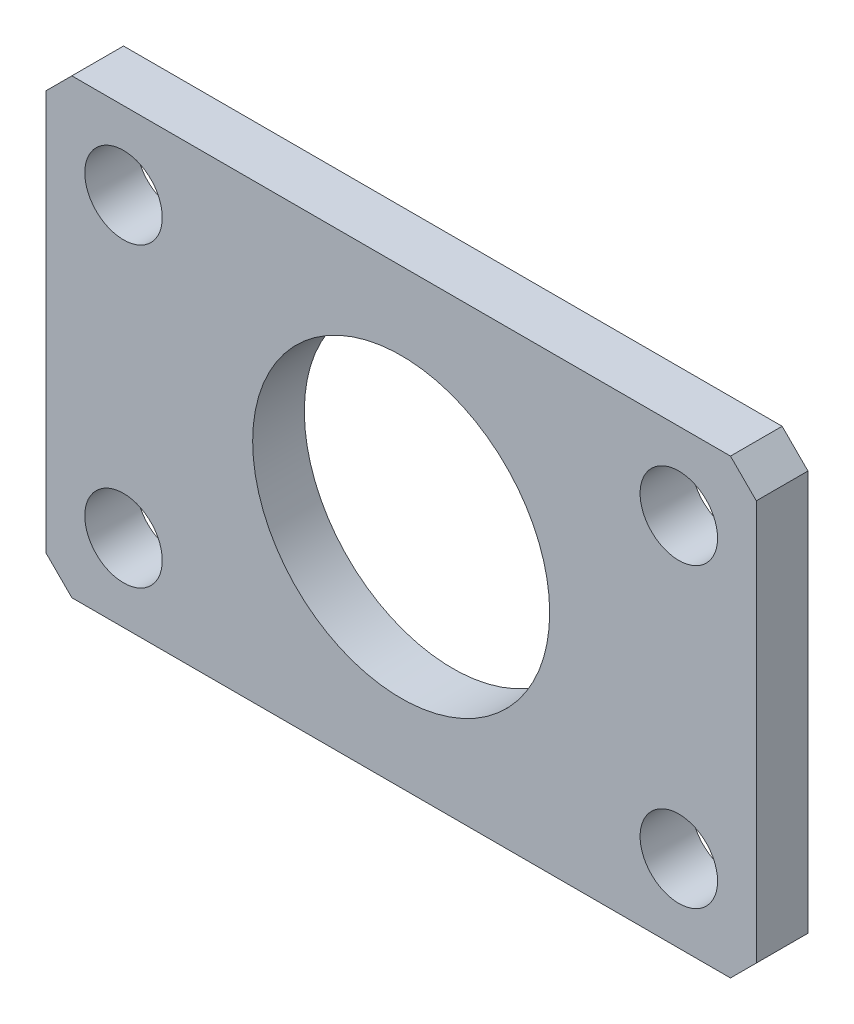
SolidWorks part; units mm, degrees
ref_plane "前视基准面" through (0, 0, 0) normal (0, 0, 1) x (1, 0, 0)
ref_plane "上视基准面" through (0, 0, 0) normal (0, 1, 0) x (1, 0, 0)
ref_plane "右视基准面" through (0, 0, 0) normal (1, 0, 0) x (0, 0, -1)
sketch "草图1" plane through (0, 0, 0) normal (0, 0, 1) x (1, 0, 0)
  line L1 (-27.5, -17.5) -> (27.5, -17.5)
  line L2 (-27.5, -17.5) -> (-27.5, 17.5)
  line L3 (-27.5, 17.5) -> (27.5, 17.5)
  line L4 (27.5, -17.5) -> (27.5, 17.5)
  line L5 (-27.5, -17.5) -> (27.5, 17.5) construction
  line L6 (-27.5, 17.5) -> (27.5, -17.5) construction
  circle A0 centre (0, 0) radius 11.5
  dimension "D1" = 23
  dimension "D2" = 55
  dimension "D3" = 35
extrude "凸台-拉伸1" add sketch "草图1" along normal mid plane 4
sketch "草图2" plane through (0, 0, 2) normal (0, 0, 1) x (1, 0, 0)
  line L0 (27.5, 17.5) -> (-27.5, 17.5) construction
  line L1 (-27.5, 17.5) -> (-27.5, -17.5) construction
  line L2 (27.5, -17.5) -> (27.5, 17.5) construction
  circle A0 centre (-21.5, 11.5) radius 3
  circle A1 centre (21.5, 11.5) radius 3
extrude "切除-拉伸1" cut sketch "草图2" against normal up to next
chamfer "倒角1" distance 2 angle 45 4 edges at (27.5, 17.5, 0) (-27.5, 17.5, 0) (27.5, -17.5, 0) (-27.5, -17.5, 0)
mirror "镜向1" about plane through (0, 0, 0) normal (0, 1, 0) of "切除-拉伸1"
equation "\"D2@草图2\"=\"D1@草图2\""
equation "\"D4@草图2\"=\"D1@草图2\""
